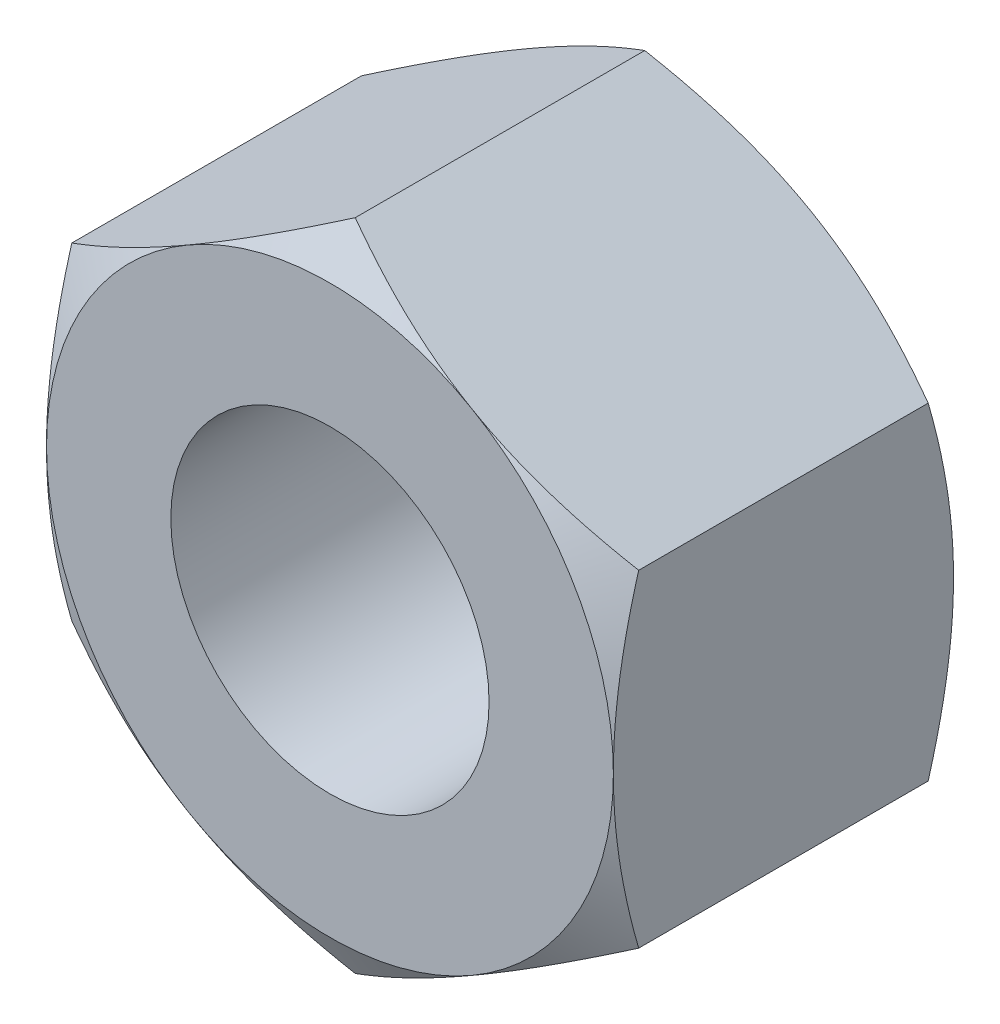
from build123d import *

# Parameters (mm, degrees)
SKETCH_1_R          = 5.0528125
EXTRUDE_597_DEPTH   = 10.8
SKETCH_2_OUTSIDE_W  = 89.934
SKETCH_2_OUTSIDE_H  = 92.718
SKETCH_2_OUTSIDE_R  = 9
CUT_EXTRUDE_1_DEPTH = 18.482562741
CUT_EXTRUDE_1_DRAFT = -60
SKETCH_3_OUTSIDE_W  = 89.934
SKETCH_3_OUTSIDE_H  = 92.718
SKETCH_3_OUTSIDE_R  = 9
CUT_EXTRUDE_2_DEPTH = 18.482562741
CUT_EXTRUDE_2_DRAFT = -60


with BuildPart() as part:
    # 草图1 → Extrude 597 (new body)
    with BuildSketch(Plane.XY):
        Polygon((0, 10.392304845), (-9, 5.196152423), (-9, -5.196152423), (0, -10.392304845), (9, -5.196152423), (9, 5.196152423), align=None)
        with Locations(Location((0, 0, 0), (0, 0, 180))):
            Circle(SKETCH_1_R, mode=Mode.SUBTRACT)
    extrude(amount=EXTRUDE_597_DEPTH)


with BuildPart() as cut_extrude_1_tool:
    # 草图2 outside → 切除-拉伸1 (with draft: the straight prism first)
    with BuildSketch(Plane(origin=(0, 0, 0), x_dir=(-1, 0, 0), z_dir=(0, 0, -1))):
        Rectangle(SKETCH_2_OUTSIDE_W, SKETCH_2_OUTSIDE_H)
        Circle(SKETCH_2_OUTSIDE_R, mode=Mode.SUBTRACT)
    extrude(amount=-CUT_EXTRUDE_1_DEPTH)
    # 切除-拉伸1: the draft: its side faces are tilted about the plane it starts from
    cut_extrude_1_sides = [cut_extrude_1_tool.faces().sort_by_distance(p)[0] for p in [
        (0, -46.359, 9.241281371),
        (-44.967, 0, 9.241281371),
        (0, 46.359, 9.241281371),
        (44.967, 0, 9.241281371),
        (9, 0, 9.241281371),
    ]]
    draft(cut_extrude_1_sides, Plane(origin=(0, 0, 0), x_dir=(-1, 0, 0), z_dir=(0, 0, -1)), CUT_EXTRUDE_1_DRAFT)


with BuildPart() as part_1:
    add(part.part)

    # 切除-拉伸1: cut by cut_extrude_1_tool
    add(cut_extrude_1_tool.part, mode=Mode.SUBTRACT)


with BuildPart() as cut_extrude_2_tool:
    # 草图3 outside → 切除-拉伸2 (with draft: the straight prism first)
    with BuildSketch(Plane.XY.offset(10.8)):
        Rectangle(SKETCH_3_OUTSIDE_W, SKETCH_3_OUTSIDE_H)
        Circle(SKETCH_3_OUTSIDE_R, mode=Mode.SUBTRACT)
    extrude(amount=-CUT_EXTRUDE_2_DEPTH)
    # 切除-拉伸2: the draft: its side faces are tilted about the plane it starts from
    cut_extrude_2_sides = [cut_extrude_2_tool.faces().sort_by_distance(p)[0] for p in [
        (0, -46.359, 1.558718629),
        (44.967, 0, 1.558718629),
        (0, 46.359, 1.558718629),
        (-44.967, 0, 1.558718629),
        (-9, 0, 1.558718629),
    ]]
    draft(cut_extrude_2_sides, Plane.XY.offset(10.8), CUT_EXTRUDE_2_DRAFT)


with BuildPart() as part_2:
    add(part_1.part)

    # 切除-拉伸2: cut by cut_extrude_2_tool
    add(cut_extrude_2_tool.part, mode=Mode.SUBTRACT)


solid = part_2.part
